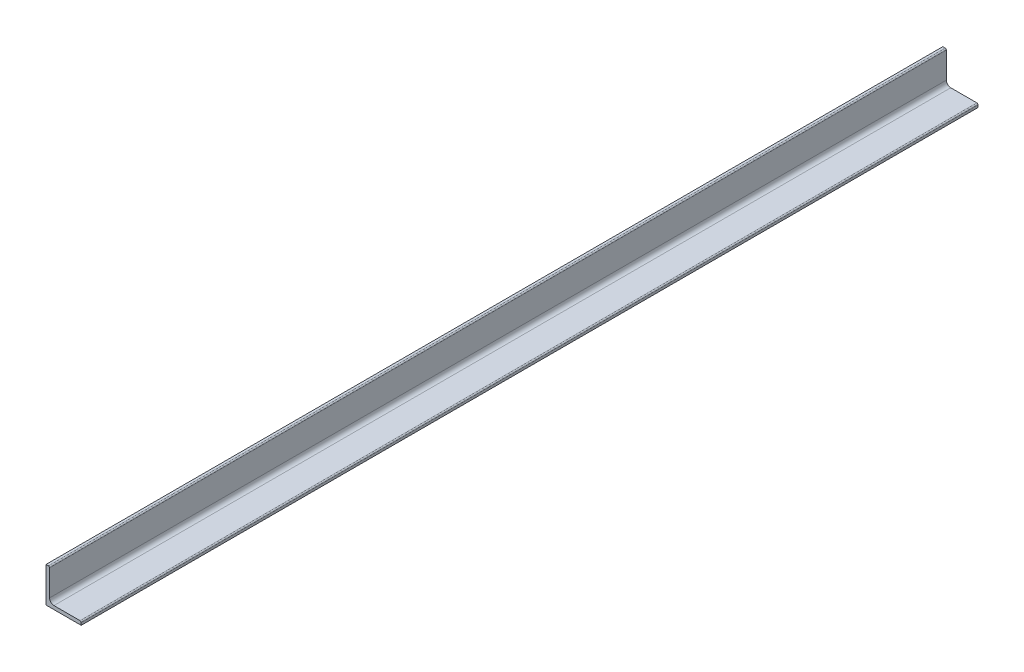
from build123d import *

# Parameters (mm, degrees)
BOSS_EXTRUDE1_DEPTH = 1020


with BuildPart() as part:
    # Sketch1 → Boss-Extrude1 (new body)
    with BuildSketch(Plane.XY):
        with BuildLine():
            Line((0, 0), (0, 40))
            Line((0, 40), (2.666666667, 40))
            ThreePointArc((2.666666667, 40), (3.609475708, 39.609475708), (4, 38.666666667))
            Line((4, 38.666666667), (4, 9))
            ThreePointArc((4, 9), (5.464466094, 5.464466094), (9, 4))
            Line((9, 4), (38.666666667, 4))
            ThreePointArc((38.666666667, 4), (39.609475708, 3.609475708), (40, 2.666666667))
            Line((40, 2.666666667), (40, 0))
            Line((40, 0), (0, 0))
        make_face()
    extrude(amount=BOSS_EXTRUDE1_DEPTH)


solid = part.part
